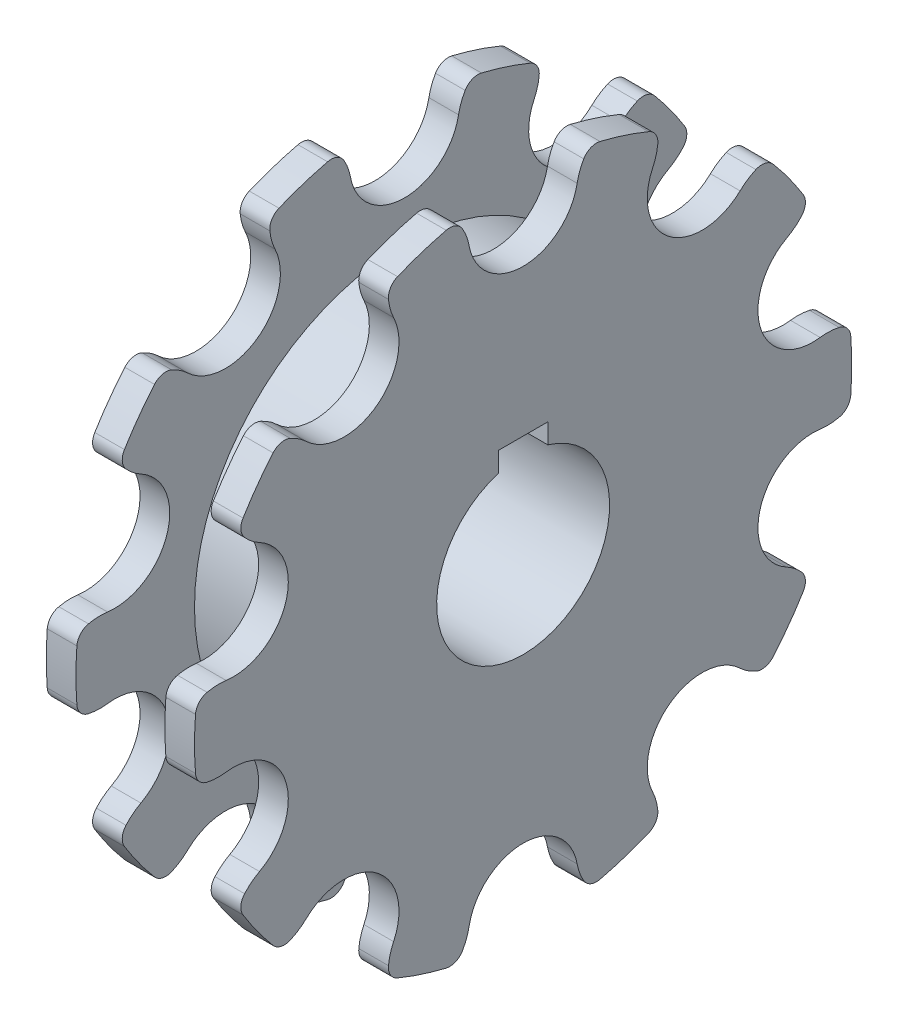
SolidWorks part; units mm, degrees
ref_plane "Front Plane" through (0, 0, 0) normal (0, 0, 1) x (1, 0, 0)
ref_plane "Top Plane" through (0, 0, 0) normal (0, 1, 0) x (1, 0, 0)
ref_plane "Right Plane" through (0, 0, 0) normal (1, 0, 0) x (0, 0, -1)
sketch "Sketch1" plane through (0, 0, 0) normal (1, 0, 0) x (0, 0, -1)
  circle A0 centre (0, 0) radius 66.5
  dimension "D1" = 133
extrude "Boss-Extrude1" add sketch "Sketch1" along normal blind 30
sketch "Sketch2" plane through (30, 0, 0) normal (1, 0, 0) x (0, 0, -1)
  circle A0 centre (0, 0) radius 17.5
  dimension "D1" = 35
extrude "Cut-Extrude1" cut sketch "Sketch2" against normal through all
sketch "Sketch3" plane through (30, 0, 0) normal (1, 0, 0) x (0, 0, -1)
  line L0 (0, 0) -> (0, 34.1948) construction
  line L3 (-5, 16.7705) -> (-5, 20.8)
  line L4 (-5, 20.8) -> (5, 20.8)
  line L5 (5, 16.7705) -> (5, 20.8)
  circle A0 centre (0, 0) radius 17.5 construction
  arc A1 (5, 16.7705) -> (-5, 16.7705) centre (0, 0) ccw
  dimension "D1" = 20.8
  dimension "D2" = 10
extrude "Cut-Extrude2" cut sketch "Sketch3" against normal through all
sketch "Sketch4" plane through (30, 0, 0) normal (1, 0, 0) x (0, 0, -1)
  line L0 (0, 0) -> (0, 61.65) construction
  circle A0 centre (0, 0) radius 61.65 construction
  arc A2 (-10.9329, 59.6461) -> (10.9329, 59.6461) centre (0, 61.65) ccw
  circle A3 centre (0, 0) radius 40 construction
  arc A5 (13.6161, 65.0911) -> (10.9329, 59.6461) centre (21.8657, 57.6421) ccw
  arc A6 (-10.9329, 59.6461) -> (-13.6161, 65.0911) centre (-21.8657, 57.6421) ccw
  arc A7 (13.6161, 65.0911) -> (-13.6161, 65.0911) centre (0, 0) ccw
  dimension "D1" = 123.3
  dimension "D2" = 80
  dimension "D3" = 22.23
  dimension "D4" = 22.23
  dimension "D5" = 22.23
  dimension "D6" = 133
extrude "Cut-Extrude3" cut sketch "Sketch4" against normal through all
fillet "Fillet1" radius 3 2 edges at (15, 65.0911, -13.6161) (15, 65.0911, 13.6161)
pattern_circular "CirPattern2" count 10 over 360 about axis through (0, 0, 0) along (1, 0, 0) of "Cut-Extrude3", "Fillet1"
sketch "Sketch5" plane through (0, 0, 0) normal (0, 1, 0) x (1, 0, 0)
  line L1 (6, 72.5) -> (24, 72.5)
  line L2 (6, 72.5) -> (6, 42.5)
  line L3 (6, 42.5) -> (24, 42.5)
  line L4 (24, 72.5) -> (24, 42.5)
  line L5 (15, -25.4128) -> (15, 6.0078) construction
  line L6 (0, -25.4128) -> (30, -25.4128) construction
  line L7 (0, 0) -> (50.8123, 0) construction
  dimension "D1" = 18
  dimension "D2" = 42.5
  dimension "D3" = 30
revolve "Cut-Revolve1" cut sketch "Sketch5" angle 360 about L7
